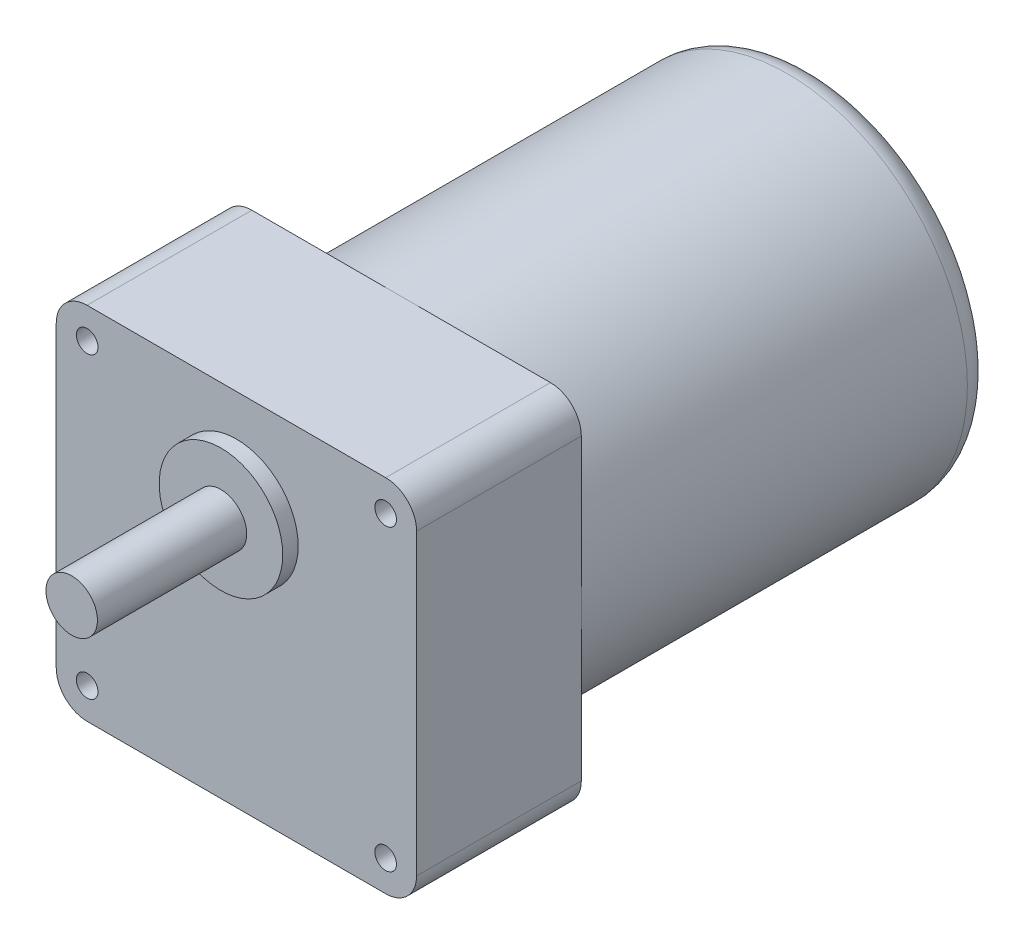
from build123d import *

# Parameters (mm, degrees)
SKETCH_1_W         = 70
SKETCH_1_H         = 70
EXTRUDE_1_DEPTH    = 32
SKETCH_2_R         = 35
EXTRUDE_2_DEPTH    = 80
FILLET_1_R         = 6
FILLET_2_R         = 5
SKETCH_3_R         = 5
EXTRUDE_3_DEPTH    = 32
HOLE_WIZARD_M5_1_D = 4.2
SKETCH_7_R         = 12
EXTRUDE_4_DEPTH    = 3


with BuildPart() as part:
    # 草图1 → 凸台-拉伸1 (new body)
    with BuildSketch(Plane.XY):
        Rectangle(SKETCH_1_W, SKETCH_1_H)
    extrude(amount=EXTRUDE_1_DEPTH)

    # 草图2 → 凸台-拉伸2 (add)
    with BuildSketch(Plane(origin=(0, 0, 0), x_dir=(-1, 0, 0), z_dir=(0, 0, -1))):
        Circle(SKETCH_2_R)
    extrude(amount=EXTRUDE_2_DEPTH)

    # 圆角1
    fillet_1_edges = [part.edges().sort_by_distance(p)[0] for p in [
        (35, -35, 16),
        (-35, -35, 16),
        (-35, 35, 16),
        (35, 35, 16),
    ]]
    fillet(fillet_1_edges, radius=FILLET_1_R)

    # 圆角2
    fillet_2_edges = [part.edges().sort_by_distance(p)[0] for p in [
        (35, 0, -80),
    ]]
    fillet(fillet_2_edges, radius=FILLET_2_R)

    # 草图3 → 凸台-拉伸3 (add)
    with BuildSketch(Plane.XY.offset(32)):
        with Locations((0, 15)):
            Circle(SKETCH_3_R)
    extrude(amount=EXTRUDE_3_DEPTH)

    # M5 螺纹孔1 (through all)
    with Locations(Plane.XY.offset(32)):
        with Locations((-28.991378029, 28.991378029), (-28.991378029, -28.991378029), (28.991378029, -28.991378029), (28.991378029, 28.991378029)):
            Hole(HOLE_WIZARD_M5_1_D / 2)

    # 草图7 → 凸台-拉伸4 (add)
    with BuildSketch(Plane.XY.offset(32)):
        with Locations((0, 15)):
            Circle(SKETCH_7_R)
    extrude(amount=EXTRUDE_4_DEPTH)


solid = part.part
